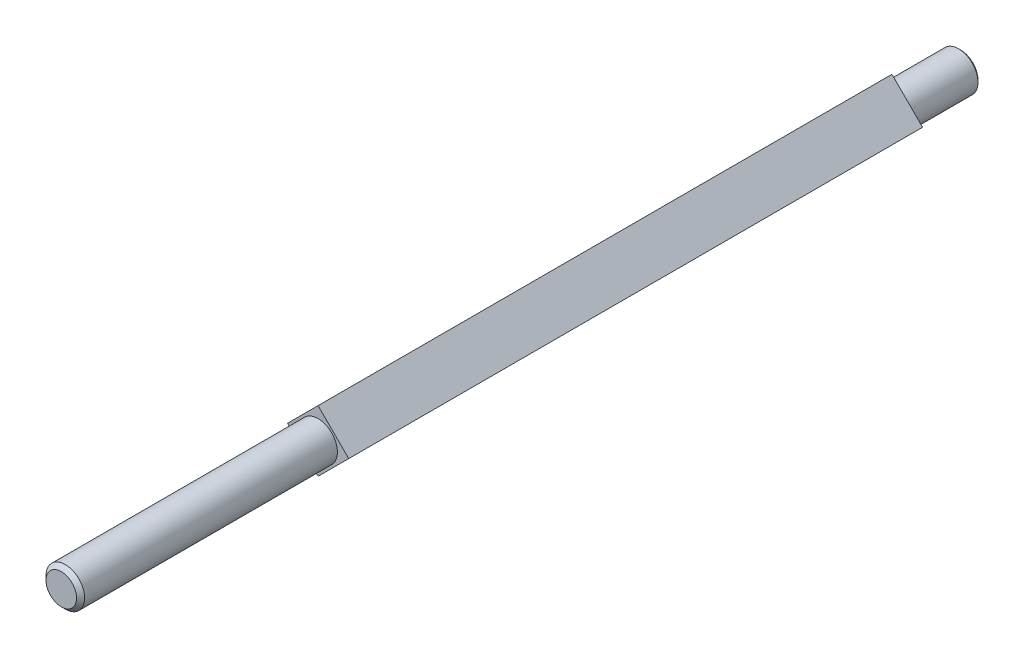
from build123d import *

# Parameters (mm, degrees)
EXTRUDE1_DEPTH = 664.7
SKETCH2_W      = 10
SKETCH2_H      = 50.8
SKETCH2_H_2    = 189.8
CHAMFER1_SIZE  = 1.5
CHAMFER2_SIZE  = 3


with BuildPart() as part:
    # Sketch1 → Extrude1 (new body)
    with BuildSketch(Plane.XY):
        Polygon((-22.627416998, 0), (0, 22.627416998), (22.627416998, 0), (0, -22.627416998), align=None)
    extrude(amount=EXTRUDE1_DEPTH)

    # Sketch2 → Cut-Revolve1 (revolve, cut)
    with BuildSketch(Plane(origin=(0, 0, 0), x_dir=(1, 0, 0), z_dir=(0, 1, 0)), mode=Mode.PRIVATE) as cut_revolve1_sk:
        with Locations((19.2875, -25.4)):
            Rectangle(SKETCH2_W, SKETCH2_H)
        with Locations((19.2875, -569.8)):
            Rectangle(SKETCH2_W, SKETCH2_H_2)
    revolve(cut_revolve1_sk.sketch.rotate(Axis((0, 0, 0), (0, 0, 1)), 180), axis=Axis((0, 0, 0), (0, 0, 1)), mode=Mode.SUBTRACT)

    # Chamfer1
    chamfer1_edges = [part.edges().sort_by_distance(p)[0] for p in [
        (14.2875, 0, 0),
    ]]
    chamfer(chamfer1_edges, length=CHAMFER1_SIZE)

    # Chamfer2
    chamfer2_edges = [part.edges().sort_by_distance(p)[0] for p in [
        (14.2875, 0, 664.7),
    ]]
    chamfer(chamfer2_edges, length=CHAMFER2_SIZE)


solid = part.part
